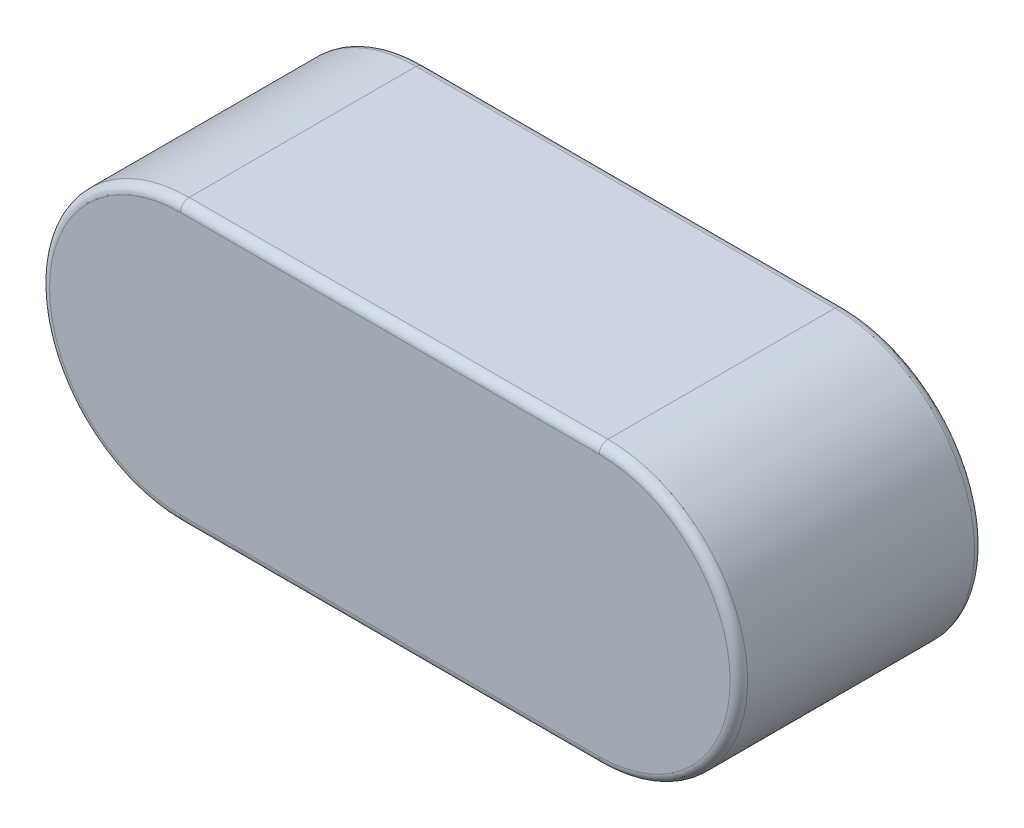
SolidWorks part; units mm, degrees
ref_plane "基准面1" through (0, 0, 0) normal (0, 0, 1) x (1, 0, 0)
ref_plane "基准面2" through (0, 0, 0) normal (0, 1, 0) x (1, 0, 0)
ref_plane "基准面3" through (0, 0, 0) normal (1, 0, 0) x (0, 0, -1)
sketch "尺寸草图" plane through (0, 0, 0) normal (0, 0, 1) x (1, 0, 0)
  line L0 (-10, 0) -> (10, 0) construction
  point P3 (-7, 0)
  point P4 (0, 0)
  point P5 (0.25, 0)
  point P8 (-8, 0)
  point P11 (0, 0)
  dimension "L" = 20
  dimension "b" = 8
  dimension "h" = 7
  dimension "r" = 0.25
sketch "草图1" plane through (0, 0, 0) normal (0, 0, 1) x (1, 0, 0)
  line L0 (-10, 0) -> (10, 0) construction
  line L1 (-6, 4) -> (6, 4)
  line L2 (-6, -4) -> (6, -4)
  line L3 (0, 2.9108) -> (0, -4) construction
  arc A0 (-6, 4) -> (-6, -4) centre (-6, 0) ccw
  arc A1 (6, 4) -> (6, -4) centre (6, 0) cw
  dimension "D3" = 20
  dimension "D1" = 4
extrude "基体-拉伸" add sketch "草图1" along normal blind 7
fillet "圆角1" radius 0.25 8 edges at (10, 0, 7) (0, 4, 7) (-10, 0, 7) (0, 4, 0) (10, 0, 0) (0, -4, 0) (-10, 0, 0) (0, -4, 7)
